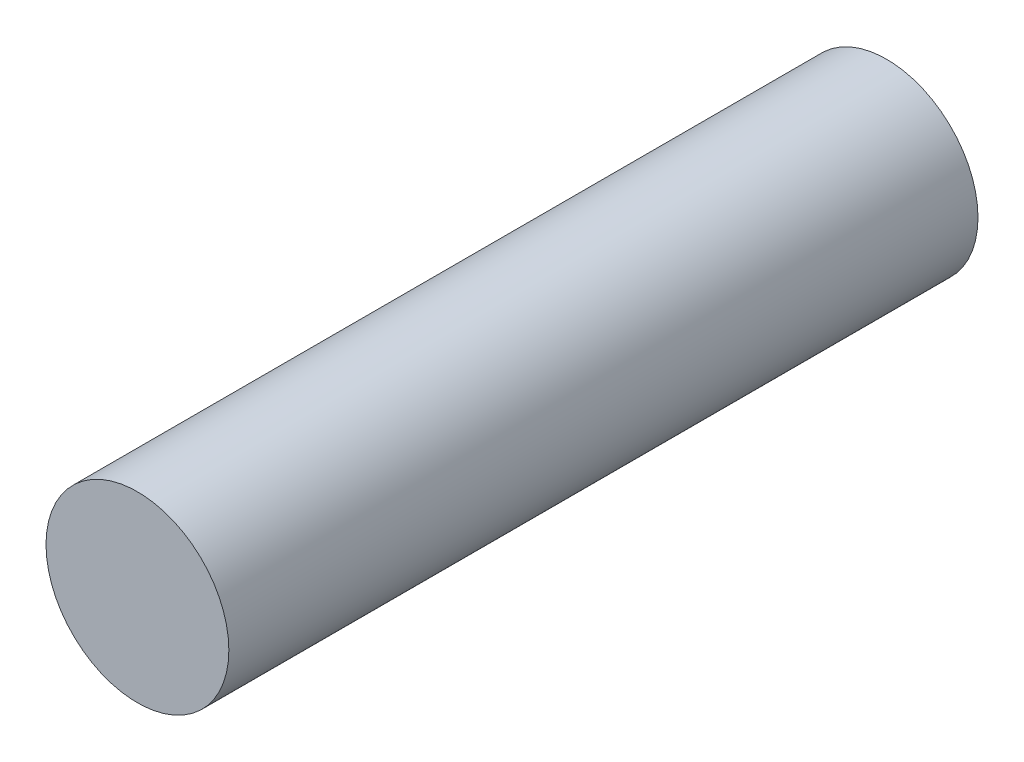
from build123d import *

# Parameters (mm, degrees)
SKETCH1_R           = 3.674588618
BOSS_EXTRUDE1_DEPTH = 30.107757446


with BuildPart() as part:
    # Sketch1 → Boss-Extrude1 (new body)
    with BuildSketch(Plane.XY):
        with Locations((-27.188857752, -16.288280471)):
            Circle(SKETCH1_R)
    extrude(amount=-BOSS_EXTRUDE1_DEPTH)


solid = part.part
